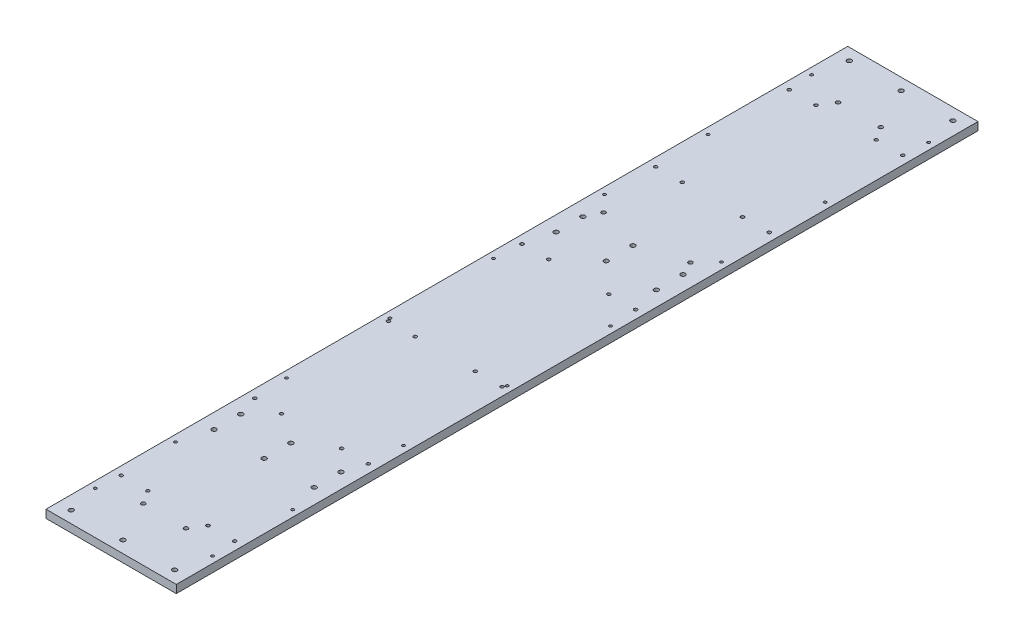
SolidWorks part; units mm, degrees
material "6061Al"
ref_plane "前视基准面" through (0, 0, 0) normal (0, 0, 1) x (1, 0, 0)
ref_plane "上视基准面" through (0, 0, 0) normal (0, 1, 0) x (1, 0, 0)
ref_plane "右视基准面" through (0, 0, 0) normal (1, 0, 0) x (0, 0, -1)
sketch "草图1" plane through (0, 0, 0) normal (0, 0, 1) x (1, 0, 0)
  line L0 (0, 0) -> (0, 30) construction
  line L1 (-97.5, 30) -> (97.5, 30)
  line L2 (97.5, 30) -> (97.5, -20)
  line L3 (-97.5, 30) -> (-97.5, -20)
  line L4 (-85.5, 18) -> (-85.5, -20)
  line L5 (-85.5, 18) -> (85.5, 18)
  line L6 (85.5, 18) -> (85.5, -20)
  line L7 (-97.5, -20) -> (-85.5, -20)
  line L8 (85.5, -20) -> (97.5, -20)
  dimension "D1" = 12
  dimension "D2" = 195
  dimension "D3" = 50
  dimension "D4" = 30
extrude "凸台-拉伸1" add sketch "草图1" along normal mid plane 1200
sketch "草图2" plane through (0, 0, -600) normal (0, 0, -1) x (-1, 0, 0)
  line L0 (97.5, 30) -> (97.5, -20) construction
  line L1 (97.5, 18) -> (-97.5, 18)
  line L2 (97.5, 18) -> (97.5, -20)
  line L3 (97.5, -20) -> (-97.5, -20)
  line L4 (-97.5, 18) -> (-97.5, -20)
  line L5 (85.5, 18) -> (-85.5, 18) construction
extrude "切除-拉伸1" cut sketch "草图2" against normal through all
hole_wizard "M6 螺纹孔1" positions "草图3" profile "草图4" tap size "M6" standard "ISO" end condition through all
sketch "草图3" plane through (0, 18, 0) normal (0, -1, 0) x (-1, 0, 0)
  line L0 (85, 500) -> (85, 300) construction
  line L1 (-45, 500) -> (-45, 300) construction
  line L2 (85, -500) -> (-45, -500) construction
  point P0 (45, 500)
  point P3 (85, 500)
  point P10 (45, 300)
  point P11 (85, 300)
  point P12 (45, 100)
  point P13 (85, 100)
  point P14 (45, -100)
  point P15 (85, -100)
  point P16 (45, -300)
  point P17 (85, -300)
  point P18 (45, -500)
  point P19 (85, -500)
  point P24 (-85, 500)
  point P25 (-45, 500)
  point P26 (-85, 300)
  point P27 (-45, 300)
  point P28 (-85, 100)
  point P29 (-45, 100)
  point P30 (-85, -100)
  point P31 (-45, -100)
  point P32 (-85, -300)
  point P33 (-45, -300)
  point P34 (-85, -500)
  point P35 (-45, -500)
  dimension "D2" = 200
  dimension "D4" = 130
  dimension "D1" = 6
  dimension "D3" = 2
sketch "草图4" plane through (-45, 18, -500) normal (1, 0, 0) x (0, 0, -1)
  line L0 (0, 0) -> (0, 12)
  line L1 (0, 12) -> (2.5, 12)
  line L2 (2.5, 12) -> (2.5, 0)
  line L5 (2.5, 0) -> (0, 0)
  line L11 (0, -6.35) -> (0, 107.95) construction
  dimension "通孔螺纹孔钻头直径" = 5
  dimension "通孔螺纹孔钻头深度" = 12
cosmetic thread "孔螺蚊线1" parameters "D2"=6
cosmetic thread "孔螺蚊线2" parameters "D2"=6
cosmetic thread "孔螺蚊线3" parameters "D2"=6
cosmetic thread "孔螺蚊线4" parameters "D2"=6
cosmetic thread "孔螺蚊线5" parameters "D2"=6
cosmetic thread "孔螺蚊线6" parameters "D2"=6
cosmetic thread "孔螺蚊线7" parameters "D2"=6
cosmetic thread "孔螺蚊线8" parameters "D2"=6
cosmetic thread "孔螺蚊线9" parameters "D2"=6
cosmetic thread "孔螺蚊线10" parameters "D2"=6
cosmetic thread "孔螺蚊线11" parameters "D2"=6
cosmetic thread "孔螺蚊线12" parameters "D2"=6
cosmetic thread "孔螺蚊线13" parameters "D2"=6
cosmetic thread "孔螺蚊线14" parameters "D2"=6
cosmetic thread "孔螺蚊线15" parameters "D2"=6
cosmetic thread "孔螺蚊线16" parameters "D2"=6
cosmetic thread "孔螺蚊线17" parameters "D2"=6
cosmetic thread "孔螺蚊线18" parameters "D2"=6
cosmetic thread "孔螺蚊线19" parameters "D2"=6
cosmetic thread "孔螺蚊线20" parameters "D2"=6
cosmetic thread "孔螺蚊线21" parameters "D2"=6
cosmetic thread "孔螺蚊线22" parameters "D2"=6
cosmetic thread "孔螺蚊线23" parameters "D2"=6
cosmetic thread "孔螺蚊线24" parameters "D2"=6
hole_wizard "M8 螺纹孔1" positions "草图5" profile "草图6" tap size "M8" standard "ISO" end condition through all
sketch "草图5" plane through (0, 30, 0) normal (0, 1, 0) x (1, 0, 0)
  point P0 (-77.5, 582.3683)
  point P3 (0, 582.3683)
  point P6 (77.5, 582.3683)
  point P9 (-77.5, -582.3683)
  point P12 (0, -582.3683)
  point P15 (77.5, -582.3683)
sketch "草图6" plane through (-77.5, 30, -582.3683) normal (1, 0, 0) x (0, 0, 1)
  line L0 (0, 0) -> (0, 12)
  line L1 (0, 12) -> (3.4, 12)
  line L2 (3.4, 12) -> (3.4, 0)
  line L5 (3.4, 0) -> (0, 0)
  line L11 (0, -6.35) -> (0, 107.95) construction
  dimension "通孔螺纹孔钻头直径" = 6.8
  dimension "通孔螺纹孔钻头深度" = 12
cosmetic thread "孔螺蚊线25" parameters "D2"=8
cosmetic thread "孔螺蚊线26" parameters "D2"=8
cosmetic thread "孔螺蚊线29" parameters "D2"=8
cosmetic thread "孔螺蚊线30" parameters "D2"=8
cosmetic thread "孔螺蚊线31" parameters "D2"=8
cosmetic thread "孔螺蚊线32" parameters "D2"=8
hole_wizard "Ø6.0mm 暗销孔1" positions "草图7" profile "草图8" hole size "Ø6.0" standard "ISO" end condition through all
sketch "草图7" plane through (0, 18, 0) normal (0, -1, 0) x (-1, 0, 0)
  line L0 (97.5, -600) -> (97.5, 600) construction
  line L1 (97.5, 600) -> (-97.5, 600) construction
  line L2 (0, 0) -> (141.474, 0) construction
  line L4 (0, 0) -> (0, 786.7909) construction
  point P0 (32, 520)
  point P18 (-32, 520)
  point P19 (-32, -520)
  point P20 (32, -520)
  dimension "D1" = 65.5
  dimension "D2" = 80
sketch "草图8" plane through (-32, 18, -520) normal (1, 0, 0) x (0, 0, -1)
  line L0 (0, 0) -> (0, 12)
  line L1 (0, 12) -> (3, 12)
  line L2 (3, 12) -> (3, 0)
  line L5 (3, 0) -> (0, 0)
  line L11 (0, -6.35) -> (0, 107.95) construction
  dimension "通孔孔直径" = 6
  dimension "通孔孔深度" = 12
hole_wizard "M5 螺纹孔1" positions "草图9" profile "草图10" tap size "M5" standard "ISO" end condition through all
sketch "草图9" plane through (0, 30, 0) normal (0, 1, 0) x (1, 0, 0)
  line L0 (0, 0) -> (0, -698.2075) construction
  circle A0 centre (-45, 500) radius 2.5 construction
  point P0 (87.6317, 536)
  point P3 (87.6317, 381)
  point P6 (87.6317, 226)
  point P9 (87.6317, 60)
  point P12 (87.6317, -95)
  point P15 (87.6317, -250)
  point P18 (87.6317, -416)
  point P21 (87.6317, -536)
  point P29 (-87.6317, -536)
  point P30 (-87.6317, -416)
  point P31 (-87.6317, -250)
  point P32 (-87.6317, -95)
  point P33 (-87.6317, 60)
  point P34 (-87.6317, 226)
  point P35 (-87.6317, 381)
  point P36 (-87.6317, 536)
  dimension "D1" = 87.6317
  dimension "D2" = 36
  dimension "D3" = 119
  dimension "D4" = 274
  dimension "D5" = 440
  dimension "D6" = 595
  dimension "D7" = 750
  dimension "D8" = 916
  dimension "D9" = 1036
sketch "草图10" plane through (87.6317, 30, -536) normal (1, 0, 0) x (0, 0, 1)
  line L0 (0, 0) -> (0, 12)
  line L1 (0, 12) -> (2.1, 12)
  line L2 (2.1, 12) -> (2.1, 0)
  line L5 (2.1, 0) -> (0, 0)
  line L11 (0, -6.35) -> (0, 107.95) construction
  dimension "通孔螺纹孔钻头直径" = 4.2
  dimension "通孔螺纹孔钻头深度" = 12
cosmetic thread "孔螺蚊线33" parameters "D2"=5
cosmetic thread "孔螺蚊线34" parameters "D2"=5
cosmetic thread "孔螺蚊线35" parameters "D2"=5
cosmetic thread "孔螺蚊线36" parameters "D2"=5
cosmetic thread "孔螺蚊线37" parameters "D2"=5
cosmetic thread "孔螺蚊线38" parameters "D2"=5
cosmetic thread "孔螺蚊线39" parameters "D2"=5
cosmetic thread "孔螺蚊线40" parameters "D2"=5
cosmetic thread "孔螺蚊线41" parameters "D2"=5
cosmetic thread "孔螺蚊线42" parameters "D2"=5
cosmetic thread "孔螺蚊线43" parameters "D2"=5
cosmetic thread "孔螺蚊线44" parameters "D2"=5
cosmetic thread "孔螺蚊线45" parameters "D2"=5
cosmetic thread "孔螺蚊线46" parameters "D2"=5
cosmetic thread "孔螺蚊线47" parameters "D2"=5
cosmetic thread "孔螺蚊线48" parameters "D2"=5
hole_wizard "M8 螺纹孔2" positions "草图11" profile "草图12" tap size "M8" standard "ISO" end condition through all
sketch "草图11" plane through (0, 30, 0) normal (0, 1, 0) x (1, 0, 0)
  line L0 (75, -371) -> (75, 141) construction
  line L1 (97.5, -600) -> (-97.5, -600) construction
  line L2 (-97.5, -600) -> (-97.5, 600) construction
  point P18 (-75, -331)
  point P21 (-75, -371)
  point P24 (0, -331)
  point P27 (0, -371)
  point P30 (75, -331)
  point P33 (75, -371)
  point P43 (-75, 181)
  point P44 (-75, 141)
  point P45 (0, 181)
  point P46 (0, 141)
  point P47 (75, 181)
  point P48 (75, 141)
  dimension "D1" = 75
  dimension "D2" = 150
  dimension "D3" = 40
  dimension "D5" = 512
  dimension "D6" = 229
  dimension "D7" = 22.5
  dimension "D4" = 2
sketch "草图12" plane through (-75, 30, 331) normal (1, 0, 0) x (0, 0, 1)
  line L0 (0, 0) -> (0, 12)
  line L1 (0, 12) -> (3.4, 12)
  line L2 (3.4, 12) -> (3.4, 0)
  line L5 (3.4, 0) -> (0, 0)
  line L11 (0, -6.35) -> (0, 107.95) construction
  dimension "通孔螺纹孔钻头直径" = 6.8
  dimension "通孔螺纹孔钻头深度" = 12
cosmetic thread "孔螺蚊线49" parameters "D2"=8
cosmetic thread "孔螺蚊线50" parameters "D2"=8
cosmetic thread "孔螺蚊线51" parameters "D2"=8
cosmetic thread "孔螺蚊线52" parameters "D2"=8
cosmetic thread "孔螺蚊线53" parameters "D2"=8
cosmetic thread "孔螺蚊线54" parameters "D2"=8
cosmetic thread "孔螺蚊线55" parameters "D2"=8
cosmetic thread "孔螺蚊线56" parameters "D2"=8
cosmetic thread "孔螺蚊线57" parameters "D2"=8
cosmetic thread "孔螺蚊线58" parameters "D2"=8
cosmetic thread "孔螺蚊线59" parameters "D2"=8
cosmetic thread "孔螺蚊线60" parameters "D2"=8
hole_wizard "Ø6.0mm 暗销孔2" positions "草图13" profile "草图14" hole size "Ø6.0" standard "ISO" end condition through all
sketch "草图13" plane through (0, 30, 0) normal (0, 1, 0) x (1, 0, 0)
  line L0 (0, 0) -> (0, 600) construction
  line L1 (97.5, 600) -> (-97.5, 600) construction
  point P0 (-65, 202)
  point P2 (65, 202)
  dimension "D1" = 398
  dimension "D2" = 130
sketch "草图14" plane through (-65, 30, -202) normal (1, 0, 0) x (0, 0, 1)
  line L0 (0, 0) -> (0, 12)
  line L1 (0, 12) -> (3, 12)
  line L2 (3, 12) -> (3, 0)
  line L5 (3, 0) -> (0, 0)
  line L11 (0, -6.35) -> (0, 107.95) construction
  dimension "通孔孔直径" = 6
  dimension "通孔孔深度" = 12
